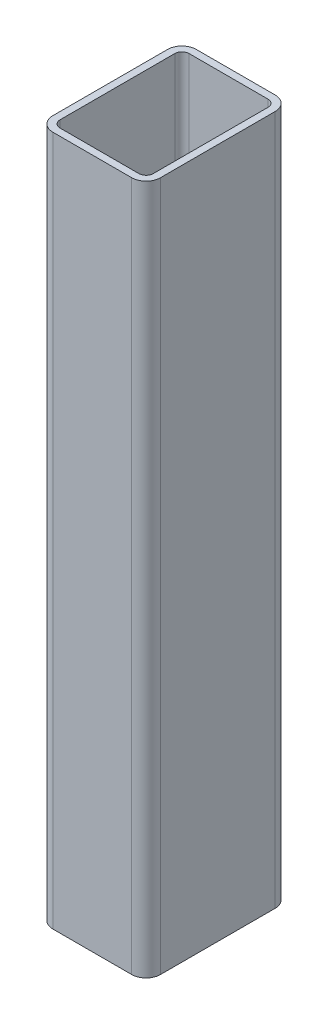
from build123d import *

# Parameters (mm, degrees)
GB_T_6728_2002_RECTANGULAR_HOLLOW_SECTIO_DEPTH = 385


with BuildPart() as part:
    # Sketch13 → GB/T 6728-2002 rectangular hollow section 80X60X4(1) (new body)
    with BuildSketch(Plane(origin=(0, 0, 0), x_dir=(-1, 0, 0), z_dir=(0, 1, 0))):
        with BuildLine():
            Line((-22, -40), (22, -40))
            ThreePointArc((22, -40), (27.656854249, -37.656854249), (30, -32))
            Line((30, -32), (30, 32))
            ThreePointArc((30, 32), (27.656854249, 37.656854249), (22, 40))
            Line((22, 40), (-22, 40))
            ThreePointArc((-22, 40), (-27.656854249, 37.656854249), (-30, 32))
            Line((-30, 32), (-30, -32))
            ThreePointArc((-30, -32), (-27.656854249, -37.656854249), (-22, -40))
        make_face()
        with BuildLine():
            Line((-22, -36), (22, -36))
            ThreePointArc((22, -36), (24.828427125, -34.828427125), (26, -32))
            Line((26, -32), (26, 32))
            ThreePointArc((26, 32), (24.828427125, 34.828427125), (22, 36))
            Line((22, 36), (-22, 36))
            ThreePointArc((-22, 36), (-24.828427125, 34.828427125), (-26, 32))
            Line((-26, 32), (-26, -32))
            ThreePointArc((-26, -32), (-24.828427125, -34.828427125), (-22, -36))
        make_face(mode=Mode.SUBTRACT)
    extrude(amount=GB_T_6728_2002_RECTANGULAR_HOLLOW_SECTIO_DEPTH)


solid = part.part
